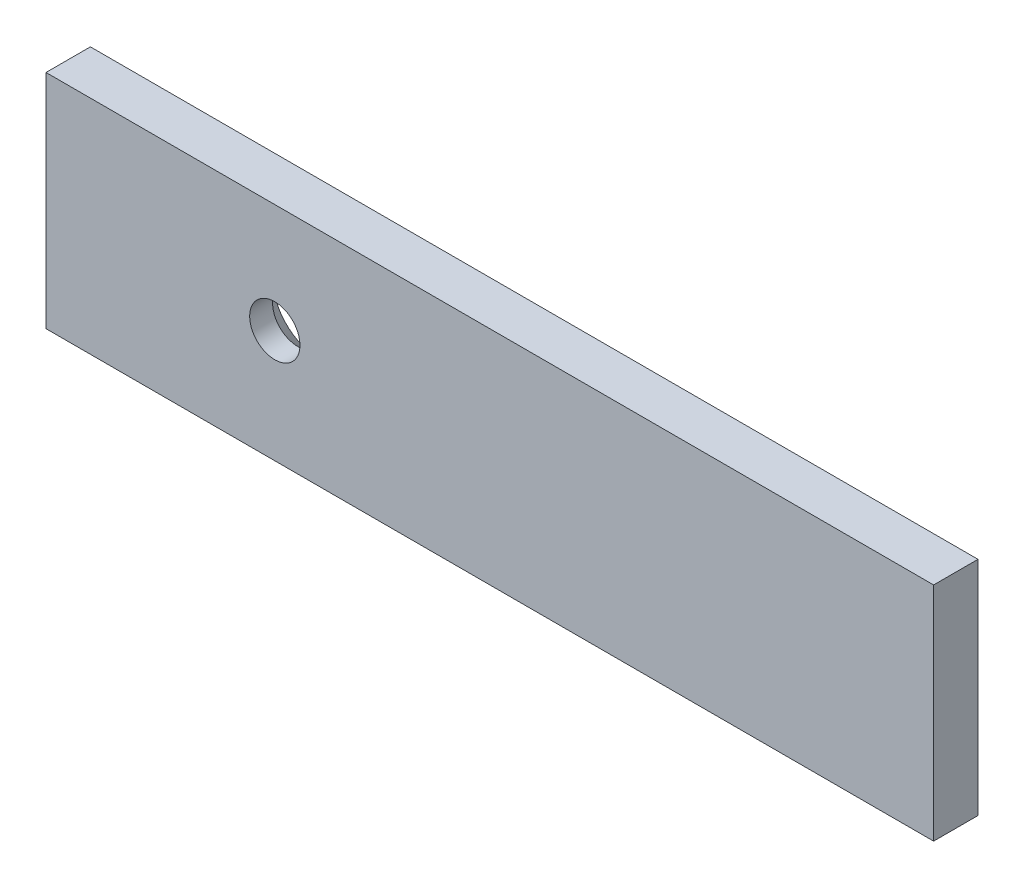
from build123d import *

# Parameters (mm, degrees)
SKETCH_1_W      = 60
SKETCH_1_H      = 15
EXTRUDE_1_DEPTH = 3


with BuildPart() as part:
    # 草图1 → 凸台-拉伸1 (new body)
    with BuildSketch(Plane.XY):
        Rectangle(SKETCH_1_W, SKETCH_1_H)
    extrude(amount=EXTRUDE_1_DEPTH)

    # 草图2 → M3 十字切槽平头螺钉锥孔1 (revolve, cut)
    with BuildSketch(Plane(origin=(-14.533919383, 0.114773803, 0), x_dir=(0, 1, 0), z_dir=(1, 0, 0))):
        Polygon((0, 0), (0, 3), (1.7, 3), (1.7, 1.45), (3.15, 0), align=None)
    revolve(axis=Axis((-14.533919383, 0.114773803, -6.35), (0, 0, 1)), mode=Mode.SUBTRACT)


solid = part.part
